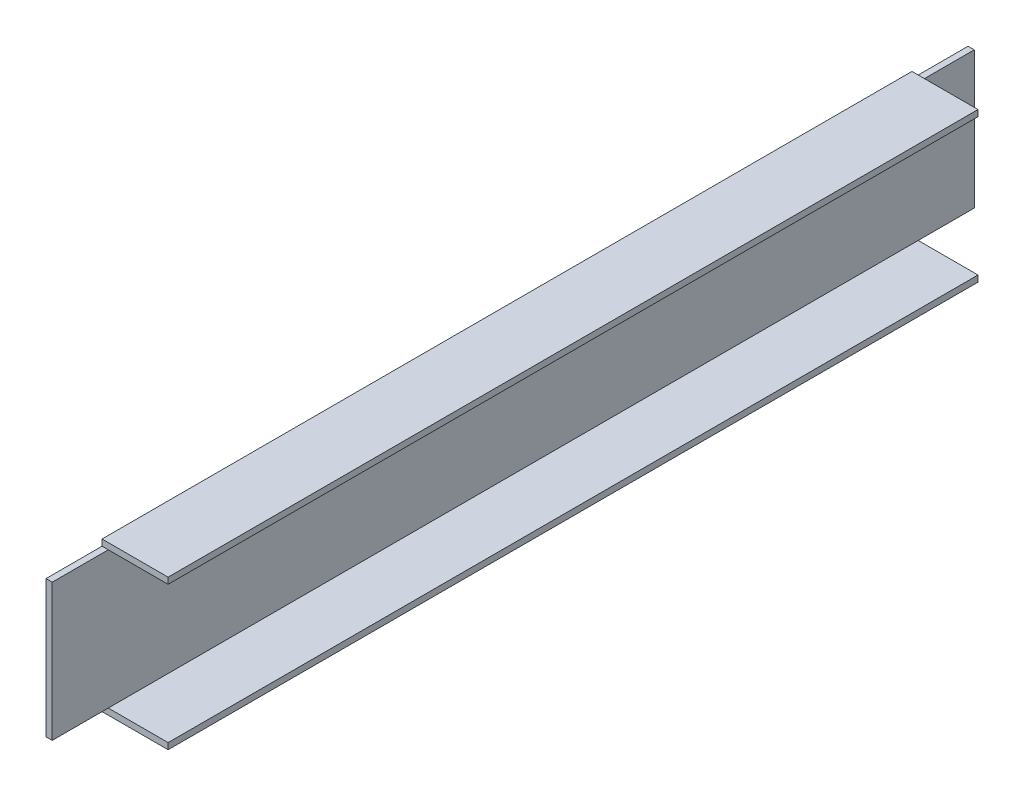
SolidWorks part; units mm, degrees
ref_plane "前视基准面" through (0, 0, 0) normal (0, 0, 1) x (1, 0, 0)
ref_plane "上视基准面" through (0, 0, 0) normal (0, 1, 0) x (1, 0, 0)
ref_plane "右视基准面" through (0, 0, 0) normal (1, 0, 0) x (0, 0, -1)
sketch "草图1" plane through (0, 0, 0) normal (0, 0, 1) x (1, 0, 0)
  line L0 (0, 0) -> (0, -120)
  line L1 (0, -120) -> (53, -120)
  line L2 (0, 0) -> (53, 0)
  line L3 (5, -5) -> (53, -5)
  line L4 (5, -5) -> (5, -115)
  line L5 (5, -115) -> (53, -115)
  line L6 (53, -5) -> (53, 0)
  line L7 (53, -120) -> (53, -115)
  dimension "D1" = 5
extrude "凸台-拉伸1" add sketch "草图1" along normal blind 740
sketch "草图2" plane through (0, 0, 0) normal (0, 0, -1) x (-1, 0, 0)
  line L0 (-53, 0) -> (0, 0)
  line L1 (0, 0) -> (0, -5)
  line L2 (0, 0) -> (0, -120) construction
  line L3 (0, -5) -> (-53, -5)
  line L4 (-53, -5) -> (-53, 0)
extrude "切除-拉伸1" cut sketch "草图2" against normal blind 45
sketch "草图3" plane through (0, 0, 0) normal (0, 0, -1) x (-1, 0, 0)
  line L0 (-53, -115) -> (0, -115)
  line L1 (0, -5) -> (0, -120) construction
  line L2 (0, -115) -> (0, -120)
  line L3 (0, -120) -> (-53, -120)
  line L4 (-53, -120) -> (-53, -115)
extrude "切除-拉伸2" cut sketch "草图3" against normal blind 45
sketch "草图4" plane through (0, 0, 740) normal (0, 0, 1) x (1, 0, 0)
  line L0 (53, -5) -> (53, 0)
  line L1 (53, 0) -> (0, 0)
  line L2 (0, 0) -> (0, -5)
  line L3 (0, 0) -> (0, -120) construction
  line L4 (0, -5) -> (53, -5)
  line L5 (53, -120) -> (0, -120)
  line L6 (53, -120) -> (53, -115)
  line L7 (53, -115) -> (0, -115)
  line L8 (0, -115) -> (0, -120)
extrude "切除-拉伸3" cut sketch "草图4" against normal blind 45
